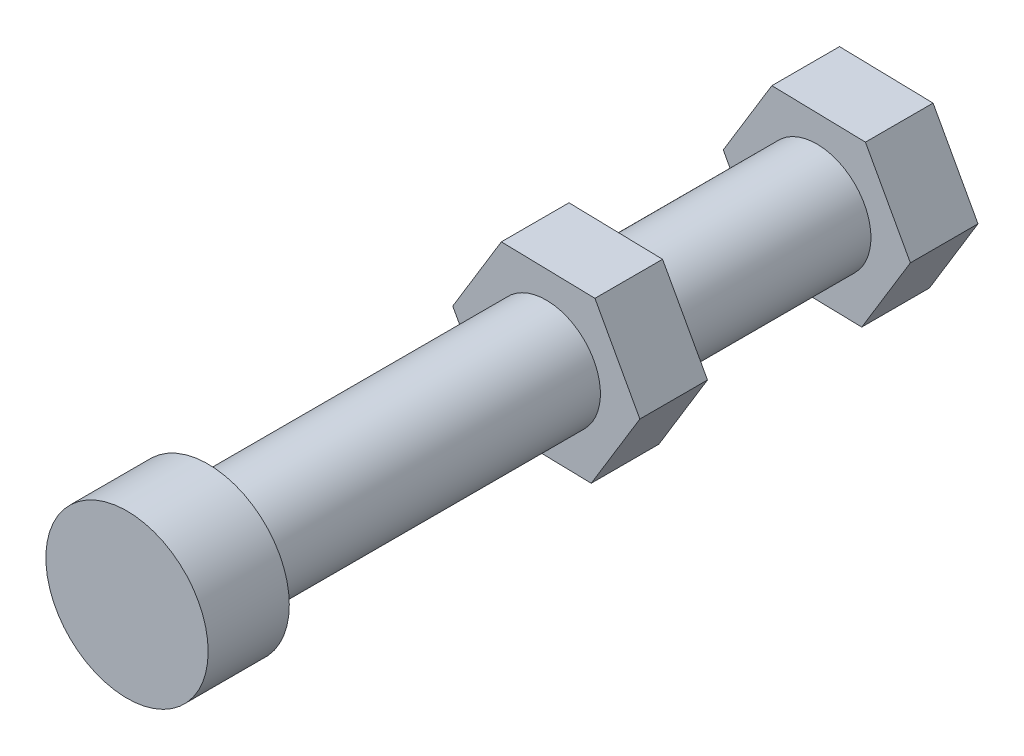
SolidWorks part; units mm, degrees
ref_plane "Front Plane" through (0, 0, 0) normal (0, 0, 1) x (1, 0, 0)
ref_plane "Top Plane" through (0, 0, 0) normal (0, 1, 0) x (1, 0, 0)
ref_plane "Right Plane" through (0, 0, 0) normal (1, 0, 0) x (0, 0, -1)
sketch "Sketch1" plane through (0, 0, 0) normal (0, 0, 1) x (1, 0, 0)
  circle A0 centre (0, 0) radius 4
  dimension "D1" = 8
extrude "Boss-Extrude1" add sketch "Sketch1" along normal blind 50
sketch "Sketch2" plane through (0, 0, 50) normal (0, 0, 1) x (1, 0, 0)
  circle A0 centre (0, 0) radius 6
  dimension "D1" = 12
extrude "Boss-Extrude2" add sketch "Sketch2" along normal blind 6
sketch "Sketch3" plane through (0, 0, 0) normal (0, 0, -1) x (-1, 0, 0)
  line L1 (3.3216, 6.0693) -> (-3.5954, 5.9112)
  line L2 (-3.5954, 5.9112) -> (-6.917, -0.1581)
  line L3 (-6.917, -0.1581) -> (-3.3216, -6.0693)
  line L4 (-3.3216, -6.0693) -> (3.5954, -5.9112)
  line L5 (3.5954, -5.9112) -> (6.917, 0.1581)
  line L6 (6.917, 0.1581) -> (3.3216, 6.0693)
  circle A0 centre (0, 0) radius 5.9918 construction
extrude "Boss-Extrude3" add sketch "Sketch3" against normal blind 5
pattern_linear "LPattern1" count 2 spacing 20 along (0, 0, 1) of "Boss-Extrude3"
